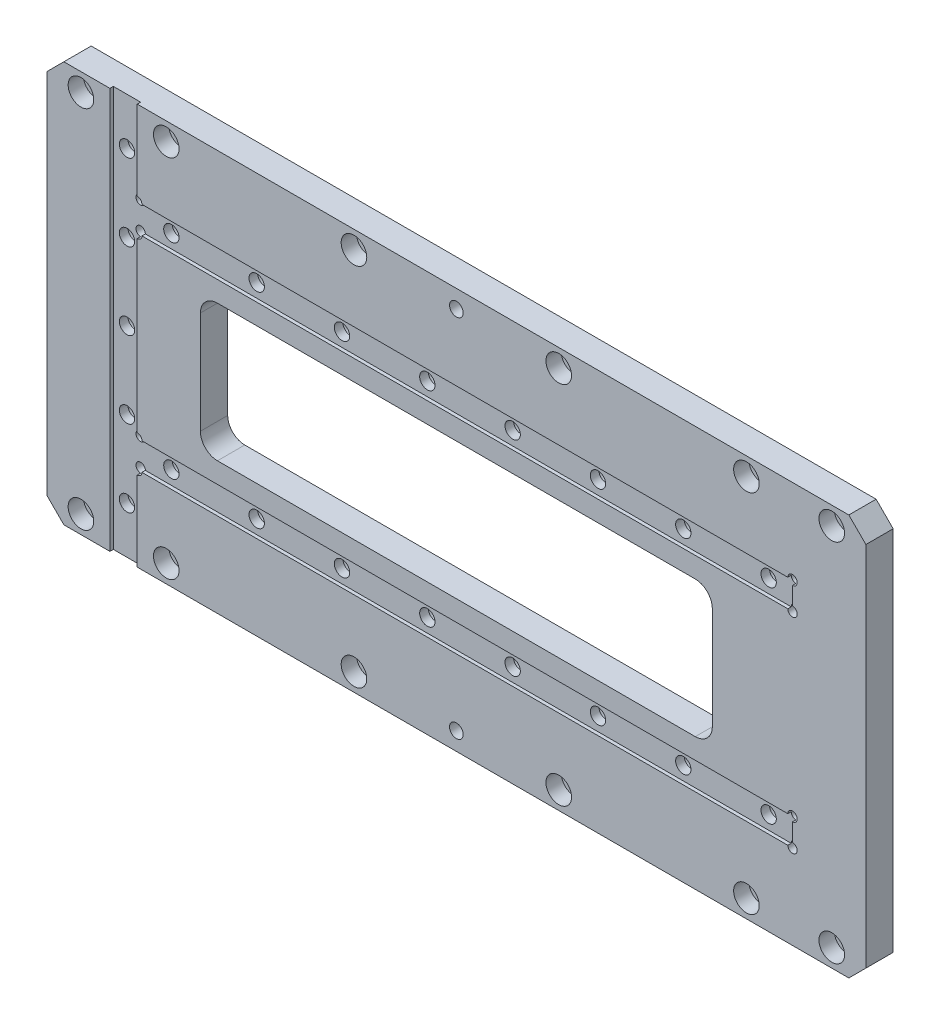
from build123d import *

# Parameters (mm, degrees)
SKETCH_1_W                  = 480
SKETCH_1_H                  = 235
EXTRUDE_1_DEPTH             = 16
HOLE_WIZARD_1_D             = 9
HOLE_WIZARD_1_CBORE_D       = 15
HOLE_WIZARD_1_CBORE_DEPTH   = 9
CHAMFER_1_SIZE              = 10
MM_1_D                      = 8
SKETCH_16_W                 = 16
SKETCH_16_H                 = 235
CUT_EXTRUDE_1_DEPTH         = 2
SKETCH_17_W                 = 400
SKETCH_17_H                 = 16
CUT_EXTRUDE_2_DEPTH         = 2
SKETCH_18_W                 = 300
SKETCH_18_H                 = 80
CUT_EXTRUDE_3_DEPTH         = 268.69805752
FILLET_1_R                  = 10
HOLE_WIZARD_3_D             = 9
HOLE_WIZARD_3_CBORE_D       = 15
HOLE_WIZARD_3_CBORE_DEPTH   = 9
HOLE_WIZARD_3_2_D           = 9
HOLE_WIZARD_3_2_CBORE_D     = 15
HOLE_WIZARD_3_2_CBORE_DEPTH = 9
PATTERN_LINEAR_1_COUNT      = 8
PATTERN_LINEAR_1_PITCH      = 50
HOLE_WIZARD_5_5_5_5_1_D     = 5.5


with BuildPart() as part:
    # 草图1 → 凸台-拉伸1 (new body)
    with BuildSketch(Plane.XY):
        Rectangle(SKETCH_1_W, SKETCH_1_H)
    extrude(amount=EXTRUDE_1_DEPTH)

    # 打孔尺寸(%根据)内六角圆柱头螺钉的类型1 (through all)
    with Locations(Plane.XY.offset(16)):
        with Locations((-220, 107), (220, -107), (-220, -107), (220, 107), (-170, 107), (-170, -107), (-60, 107), (-60, -107), (60, 107), (60, -107), (170, 107), (170, -107)):
            CounterBoreHole(HOLE_WIZARD_1_D / 2, HOLE_WIZARD_1_CBORE_D / 2, HOLE_WIZARD_1_CBORE_DEPTH)

    # 倒角1
    chamfer_1_edges = [part.edges().sort_by_distance(p)[0] for p in [
        (-240, 117.5, 8),
        (240, 117.5, 8),
        (240, -117.5, 8),
        (-240, -117.5, 8),
    ]]
    chamfer(chamfer_1_edges, length=CHAMFER_1_SIZE)

    # 大小mm 暗销孔1 (through all)
    with Locations(Plane.XY.offset(16)):
        with Locations((0, -107), (0, 107)):
            Hole(MM_1_D / 2)

    # 草图16 → 切除-拉伸1 (cut)
    with BuildSketch(Plane.XY.offset(16)):
        with Locations((-195, 0)):
            Rectangle(SKETCH_16_W, SKETCH_16_H)
    extrude(amount=-CUT_EXTRUDE_1_DEPTH, mode=Mode.SUBTRACT)

    # 草图17 → 切除-拉伸2 (cut)
    with BuildSketch(Plane.XY.offset(16)):
        with Locations((-3, -60)):
            Rectangle(SKETCH_17_W, SKETCH_17_H)
        with Locations((-3, 60)):
            Rectangle(SKETCH_17_W, SKETCH_17_H)
    extrude(amount=-CUT_EXTRUDE_2_DEPTH, mode=Mode.SUBTRACT)

    # 草图18 → 切除-拉伸3 (cut, through all)
    with BuildSketch(Plane.XY.offset(16)):
        Rectangle(SKETCH_18_W, SKETCH_18_H)
    extrude(amount=-CUT_EXTRUDE_3_DEPTH, mode=Mode.SUBTRACT)

    # 圆角1
    fillet_1_edges = [part.edges().sort_by_distance(p)[0] for p in [
        (150, 40, 8),
        (150, -40, 8),
        (-150, -40, 8),
        (-150, 40, 8),
    ]]
    fillet(fillet_1_edges, radius=FILLET_1_R)

    # Hole Wizard 3 (through all)
    with Locations(Plane(origin=(0, 0, 0), x_dir=(-1, 0, 0), z_dir=(0, 0, -1))):
        with Locations((195, 0), (195, 45), (195, 90), (195, -90), (195, -45)):
            CounterBoreHole(HOLE_WIZARD_3_D / 2, HOLE_WIZARD_3_CBORE_D / 2, HOLE_WIZARD_3_CBORE_DEPTH)

    # Hole Wizard 3 2 (through all)
    with Locations(Plane(origin=(0, 0, 0), x_dir=(-1, 0, 0), z_dir=(0, 0, -1))):
        with Locations((169, -60), (169, 60)):
            hole_wizard_3_2 = CounterBoreHole(HOLE_WIZARD_3_2_D / 2, HOLE_WIZARD_3_2_CBORE_D / 2, HOLE_WIZARD_3_2_CBORE_DEPTH)

    # 阵列(线性)1: Hole Wizard 3 2 ×8
    with Locations(*[(i * PATTERN_LINEAR_1_PITCH, 0, 0) for i in range(1, PATTERN_LINEAR_1_COUNT)]):
        add(hole_wizard_3_2, mode=Mode.SUBTRACT)

    # Ø5.5 (5.5) 直径孔1 (through all)
    with Locations(Plane.XY.offset(16)):
        with Locations((197, -68), (197, -52), (197, 52), (197, 68), (-187, 68), (-187, 52), (-187, -68), (-187, -52)):
            Hole(HOLE_WIZARD_5_5_5_5_1_D / 2)


solid = part.part
